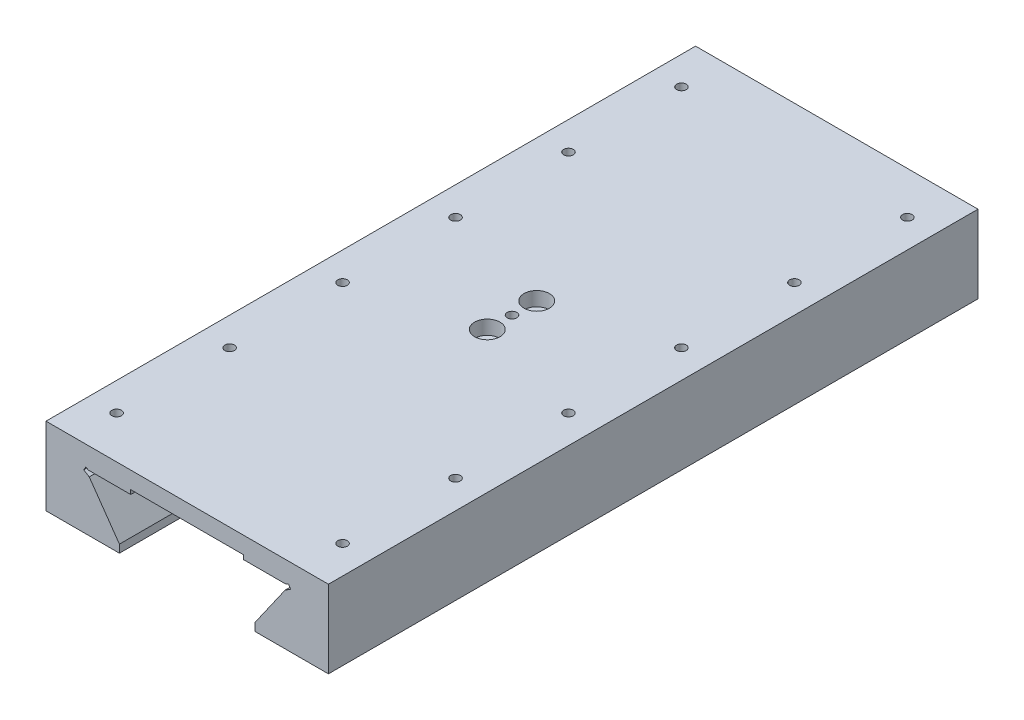
SolidWorks part; units mm, degrees
ref_plane "Front Plane" through (0, 0, 0) normal (0, 0, 1) x (1, 0, 0)
ref_plane "Top Plane" through (0, 0, 0) normal (0, 1, 0) x (1, 0, 0)
ref_plane "Right Plane" through (0, 0, 0) normal (1, 0, 0) x (0, 0, -1)
sketch "Sketch1" plane through (0, 0, 0) normal (0, 0, 1) x (1, 0, 0)
  line L2 (0, 30.5) -> (0, 93.1667) construction
  line L3 (-40, 52.5) -> (-40, 55.5)
  line L4 (-40, 55.5) -> (40, 55.5)
  line L5 (-40, 52.5) -> (-70, 52.5)
  line L6 (-100, 12.5) -> (-48, 12.5)
  line L7 (-47.7029, 12.5) -> (-104, 12.5) construction
  line L8 (-48, 12.5) -> (-48, 18.0807)
  line L9 (-70, 49.5) -> (-45.5683, 14.6079) construction
  line L10 (-48, 18.0807) -> (-69.3858, 48.6228)
  line L11 (-100, 12.5) -> (-100, 67.5)
  line L12 (-100, 67.5) -> (100, 67.5)
  line L13 (-5, 52.5) -> (-70, 52.5) construction
  line L14 (-70, 52.5) -> (-71.7114, 53.5349)
  line L15 (-71.7114, 53.5349) -> (-73.2637, 50.9677)
  line L16 (-73.2637, 50.9677) -> (-69.3858, 48.6228)
  line L17 (73.2637, 50.9677) -> (69.3858, 48.6228)
  line L18 (71.7114, 53.5349) -> (73.2637, 50.9677)
  line L19 (70, 52.5) -> (71.7114, 53.5349)
  line L20 (100, 12.5) -> (100, 67.5)
  line L21 (48, 18.0807) -> (69.3858, 48.6228)
  line L22 (48, 12.5) -> (48, 18.0807)
  line L23 (100, 12.5) -> (48, 12.5)
  line L24 (40, 52.5) -> (70, 52.5)
  line L25 (40, 52.5) -> (40, 55.5)
  point P9 (-48, 15.2904)
  point P34 (0, 67.5)
  point P39 (0, 55.5)
  dimension "D1" = 48
  dimension "D2" = 100
  dimension "D3" = 3
  dimension "D4" = 3
  dimension "D5" = 2
  dimension "D6" = 55
extrude "Boss-Extrude1" add sketch "Sketch1" against normal up to surface (460 mm away)
hole_wizard "CBORE for M8 Hex Head Bolt1" positions "Sketch4" profile "Sketch5" counterbore size "M8" standard "GB" end condition up to next
sketch "Sketch4" plane through (0, 67.5, 0) normal (0, 1, 0) x (1, 0, 0)
  line L0 (-100, 230) -> (100, 230) construction
  line L1 (-100, 460) -> (-100, 0) construction
  line L2 (100, 460) -> (100, 0) construction
  point P0 (0, 247.5)
  point P2 (0, 212.5)
  dimension "D1" = 35
sketch "Sketch5" plane through (0, 67.5, -247.5) normal (1, 0, 0) x (0, 0, 1)
  line L0 (0, 0) -> (0, 12)
  line L1 (0, 12) -> (4.5, 12)
  line L3 (4.5, 12) -> (4.5, 10)
  line L4 (4.5, 10) -> (9, 10)
  line L5 (9, 10) -> (9, 0)
  line L7 (9, 0) -> (0, 0)
  line L11 (0, -6.35) -> (0, 107.95) construction
  dimension "通孔孔直径" = 9
  dimension "通孔孔深度" = 12
  dimension "柱形沉头孔直径" = 18
  dimension "柱形沉头孔深度" = 10
hole_wizard "M8 Tapped Hole1" positions "Sketch6" profile "Sketch7" tap size "M8" standard "GB"
sketch "Sketch6" plane through (0, 67.5, 0) normal (0, 1, 0) x (1, 0, 0)
  line L0 (0, 460) -> (0, 0) construction
  line L1 (-100, 460) -> (100, 460) construction
  line L3 (-100, 230) -> (100, 230) construction
  line L4 (-100, 460) -> (-100, 0) construction
  line L5 (100, 460) -> (100, 0) construction
  line L8 (-80, 30) -> (80, 30) construction
  line L9 (-80, 30) -> (-80, 430) construction
  line L10 (-80, 430) -> (80, 430) construction
  line L11 (80, 30) -> (80, 430) construction
  line L12 (-80, 30) -> (80, 430) construction
  line L13 (-80, 430) -> (80, 30) construction
  line L14 (-80, 350) -> (80, 350) construction
  line L16 (-80, 270) -> (80, 270) construction
  line L18 (-80, 190) -> (80, 190) construction
  line L20 (-80, 110) -> (80, 110) construction
  point P15 (0, 230)
  point P16 (80, 430)
  point P199 (-80, 30)
  point P200 (-80, 430)
  point P201 (80, 30)
  point P204 (-80, 350)
  point P205 (80, 350)
  point P208 (-80, 270)
  point P209 (80, 270)
  point P212 (-80, 190)
  point P213 (80, 190)
  point P216 (-80, 110)
  point P217 (80, 110)
  dimension "D1" = 30
  dimension "D2" = 80
  dimension "D3" = 80
  dimension "D4" = 80
  dimension "D5" = 80
  dimension "D6" = 20
sketch "Sketch7" plane through (0, 67.5, -230) normal (1, 0, 0) x (0, 0, 1)
  line L0 (0, 0) -> (0, 21.7929)
  line L1 (0, 21.7929) -> (3.4, 19.75)
  line L2 (3.4, 19.75) -> (3.4, 0)
  line L5 (3.4, 0) -> (0, 0)
  line L10 (0, 21.7929) -> (-3.4, 19.75) construction
  line L11 (0, -6.35) -> (0, 107.95) construction
  dimension "螺纹孔钻头直径" = 6.8
  dimension "螺纹孔钻头深度" = 19.75
  dimension "导头角度" = 118
cosmetic thread "Cosmetic Thread1" parameters "D1"=16, "D2"=8
cosmetic thread "Cosmetic Thread2" parameters "D1"=16, "D2"=8
cosmetic thread "Cosmetic Thread3" parameters "D1"=16, "D2"=8
cosmetic thread "Cosmetic Thread4" parameters "D1"=16, "D2"=8
cosmetic thread "Cosmetic Thread5" parameters "D1"=16, "D2"=8
cosmetic thread "Cosmetic Thread6" parameters "D1"=16, "D2"=8
cosmetic thread "Cosmetic Thread7" parameters "D1"=16, "D2"=8
cosmetic thread "Cosmetic Thread8" parameters "D1"=16, "D2"=8
cosmetic thread "Cosmetic Thread9" parameters "D1"=16, "D2"=8
cosmetic thread "Cosmetic Thread10" parameters "D1"=16, "D2"=8
cosmetic thread "Cosmetic Thread11" parameters "D1"=16, "D2"=8
cosmetic thread "Cosmetic Thread12" parameters "D1"=16, "D2"=8
cosmetic thread "Cosmetic Thread13" parameters "D1"=12, "D2"=8
